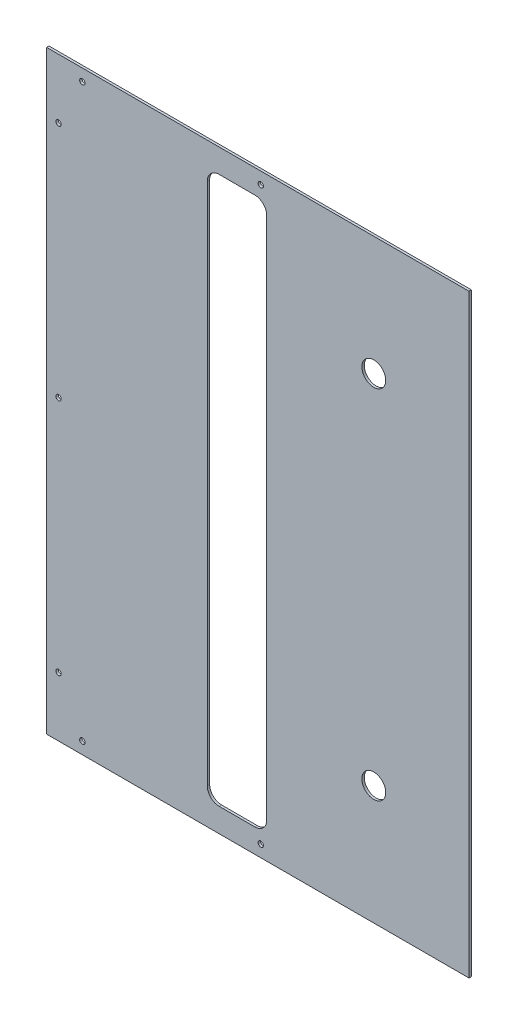
from build123d import *

# Parameters (mm, degrees)
SKETCH_1_W                  = 355
SKETCH_1_H                  = 500
EXTRUDE_1_DEPTH             = 2
HOLE_WIZARD_4_5_4_5_1_D     = 4.5
HOLE_WIZARD_4_5_4_5_1_DEPTH = 8
HOLE_WIZARD_4_5_4_5_1_TIP   = 1.351936393
SKETCH_4_W                  = 50
SKETCH_4_H                  = 460
CUT_EXTRUDE_1_DEPTH         = 10
FILLET_1_R                  = 10
SKETCH_5_R                  = 10
CUT_EXTRUDE_2_DEPTH         = 10


with BuildPart() as part:
    # 草图1 → 凸台-拉伸1 (new body)
    with BuildSketch(Plane.XY):
        Rectangle(SKETCH_1_W, SKETCH_1_H)
    extrude(amount=EXTRUDE_1_DEPTH)

    # Ø4.5 (4.5) 直径孔1
    with Locations(Plane.XY.offset(2)):
        with Locations((-147.5, -240), (-167.5, 0), (-167.5, 200), (-167.5, -200), (-147.5, 240), (2.5, 240), (2.5, -240)):
            Hole(HOLE_WIZARD_4_5_4_5_1_D / 2, depth=HOLE_WIZARD_4_5_4_5_1_DEPTH)
            with Locations((0, 0, -(HOLE_WIZARD_4_5_4_5_1_DEPTH + HOLE_WIZARD_4_5_4_5_1_TIP / 2))):  # 118° drill point
                Cone(0, HOLE_WIZARD_4_5_4_5_1_D / 2, HOLE_WIZARD_4_5_4_5_1_TIP, mode=Mode.SUBTRACT)

    # 草图4 → 切除-拉伸1 (cut)
    with BuildSketch(Plane(origin=(0, 0, 0), x_dir=(-1, 0, 0), z_dir=(0, 0, -1))):
        with Locations((17.5, 0)):
            Rectangle(SKETCH_4_W, SKETCH_4_H)
    extrude(amount=-CUT_EXTRUDE_1_DEPTH, mode=Mode.SUBTRACT)

    # 圆角1
    fillet_1_edges = [part.edges().sort_by_distance(p)[0] for p in [
        (-42.5, 230, 1),
        (-42.5, -230, 1),
        (7.5, -230, 1),
        (7.5, 230, 1),
    ]]
    fillet(fillet_1_edges, radius=FILLET_1_R)

    # 草图5 → 切除-拉伸2 (cut)
    with BuildSketch(Plane(origin=(0, 0, 0), x_dir=(-1, 0, 0), z_dir=(0, 0, -1))):
        with Locations((-97.5, -150)):
            Circle(SKETCH_5_R)
        with Locations((-97.5, 150)):
            Circle(SKETCH_5_R)
    extrude(amount=-CUT_EXTRUDE_2_DEPTH, mode=Mode.SUBTRACT)


solid = part.part
